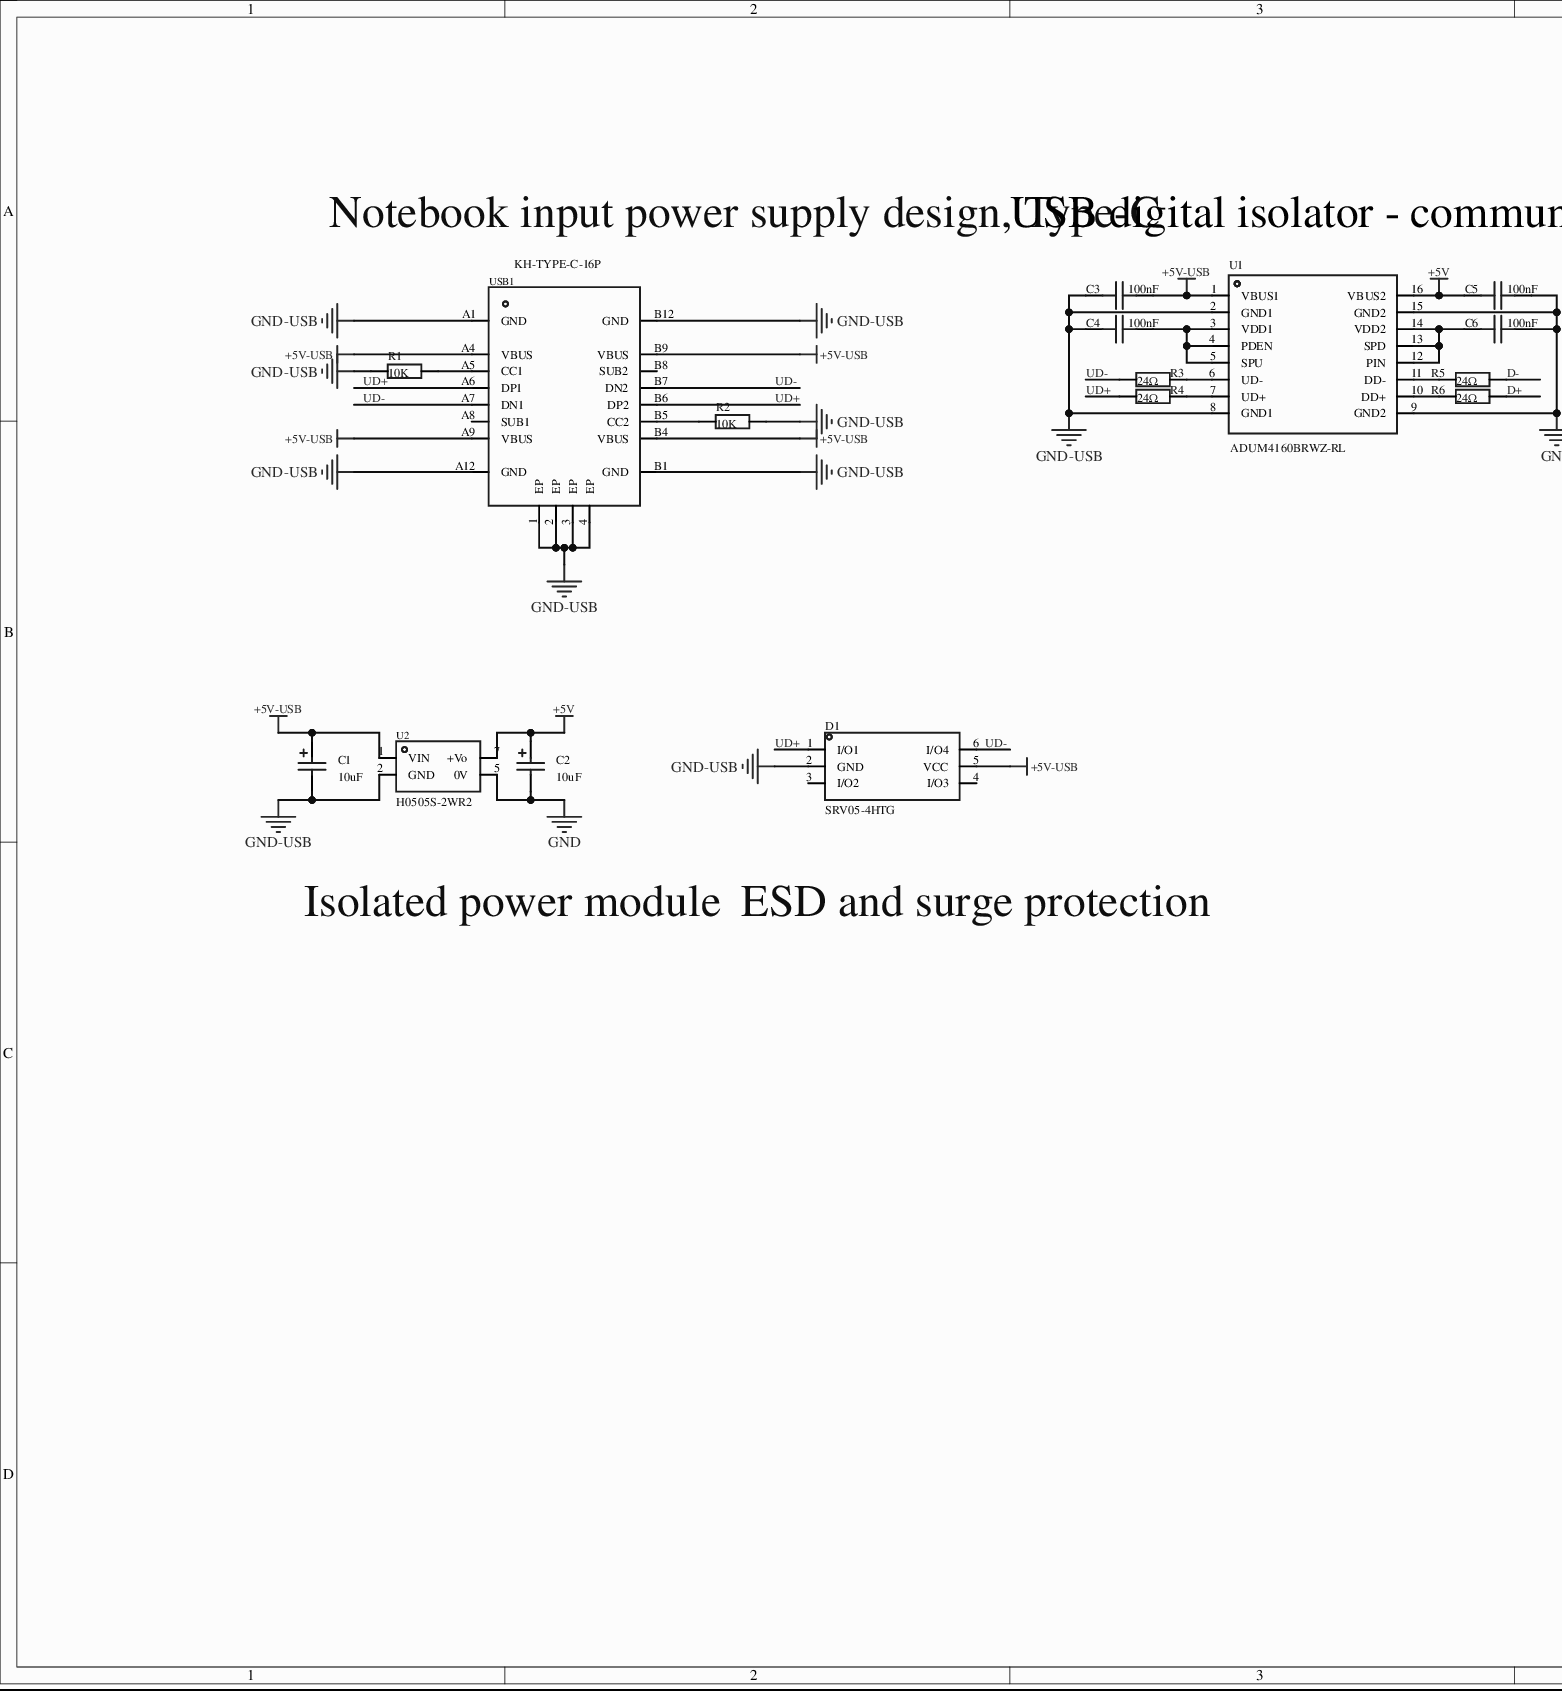
[diagram p0: MISC79005-3.schdoc, left]
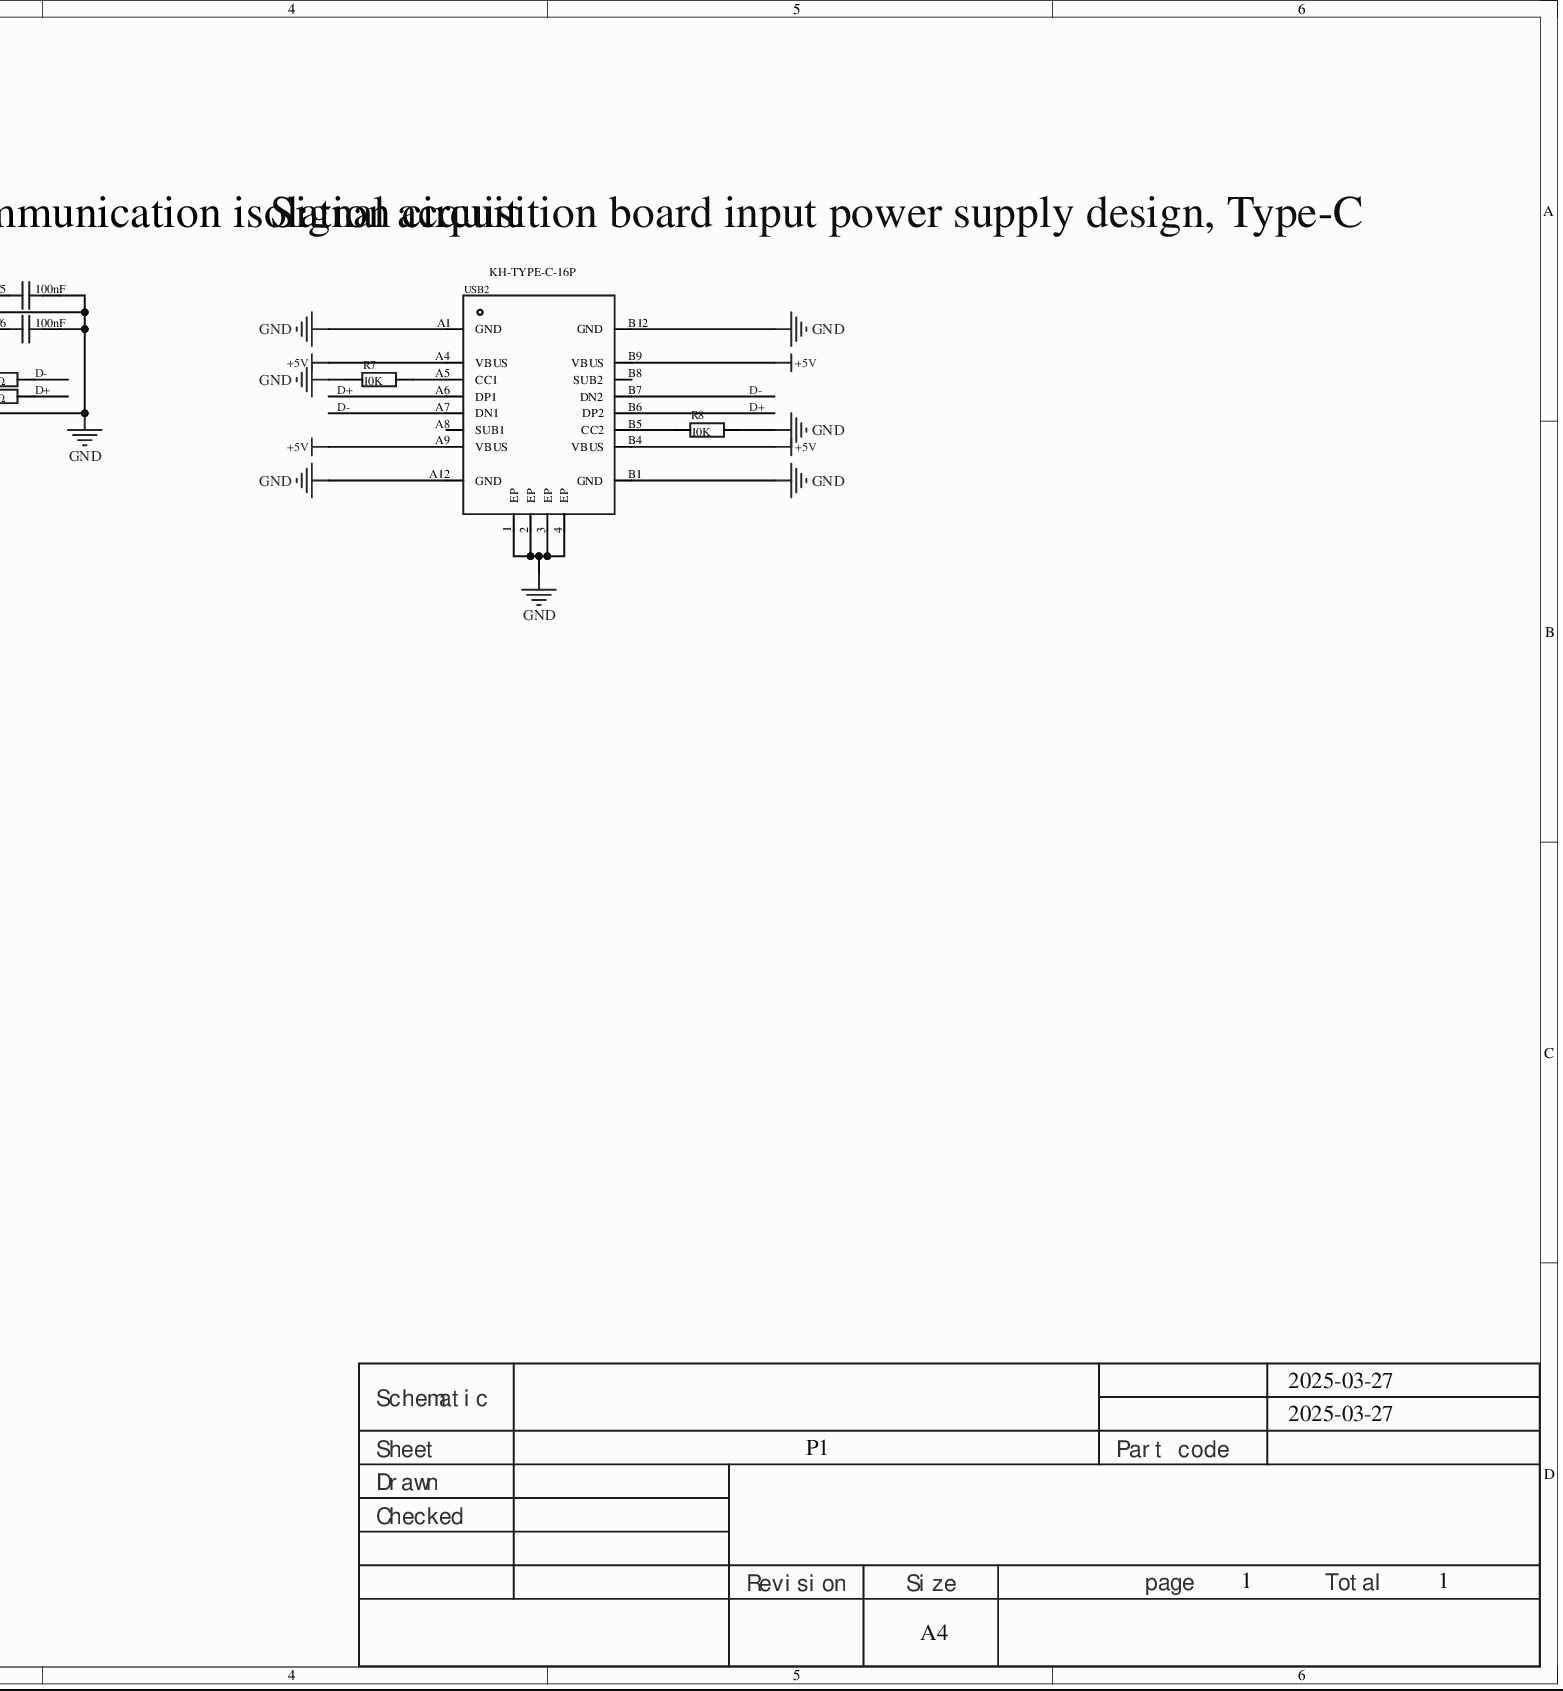
[diagram p1: MISC79005-3.schdoc, right]
# Altium project MISC79005-2.PrjPcb
1 sheet, 19 parts. Net scope: global (net labels, ports and power ports of the same name join across sheets).
Board file: MISC79005.pcbdoc

## Sheet MISC79005-3.schdoc
size 457 x 254 mm; Version: V1.0; @Project Name: MISC79005; @Page Count: 1; @Update Date: 2025-03-27; @Create Date: 2025-03-27; @Schematic Name: MISC79005; @Page No: 1; @Board Name: MISC79005; @Create Time: 09:58:40; @Update Time: 21:52:18

### Parts
C1  10uF  [CAP-SMD_L3.2-W1.6-RD-C7171]
C2  10uF  [CAP-SMD_L3.2-W1.6-RD-C7171]
C3  100nF  [C0603]
C4  100nF  [C0603]
C5  100nF  [C0603]
C6  100nF  [C0603]
D1  SRV05-4HTG  [SOT-23-6_L2.9-W1.6-P0.95-LS2.8-BL]
R1  10K  [R0603]
R2  10K  [R0603]
R3  24Ω  [R0603]
R4  24Ω  [R0603]
R5  24Ω  [R0603]
R6  24Ω  [R0603]
R7  10K  [R0603]
R8  10K  [R0603]
U1  ADUM4160BRWZ-RL  [SOIC-16_L10.3-W7.5-P1.27-LS10.3-BL]
U2  H0505S-2WR2  [PWRM-TH_EVISUN_HXXXXS-2WR2]
USB1  KH-TYPE-C-16P  [USB-C-SMD_KH-TYPE-C-16P]
USB2  KH-TYPE-C-16P  [USB-C-SMD_KH-TYPE-C-16P]

### Nets
+5V: C2.1 C5.1 U1.16(VBUS2) U2.7(+Vo) USB2.A4(VBUS) USB2.A9(VBUS) USB2.B4(VBUS) USB2.B9(VBUS)
+5V-USB: C1.1 C3.2 D1.5(VCC) U1.1(VBUS1) U2.1(VIN) USB1.A4(VBUS) USB1.A9(VBUS) USB1.B4(VBUS) USB1.B9(VBUS)
GND: C2.2 C5.2 C6.2 R7.2 R8.1 U1.9(GND2) U1.15(GND2) U2.5(0V) USB2.1(EP) USB2.2(EP) USB2.3(EP) USB2.4(EP) USB2.A1(GND) USB2.A12(GND) USB2.B1(GND) USB2.B12(GND)
GND-USB: C1.2 C3.1 C4.1 D1.2(GND) R1.2 R2.1 U1.2(GND1) U1.8(GND1) U2.2(GND) USB1.1(EP) USB1.2(EP) USB1.3(EP) USB1.4(EP) USB1.A1(GND) USB1.A12(GND) USB1.B1(GND) USB1.B12(GND)
D+: R6.2 USB2.A6(DP1) USB2.B6(DP2)
D-: R5.2 USB2.A7(DN1) USB2.B7(DN2)
UD+: D1.1(I/O1) R4.1 USB1.A6(DP1) USB1.B6(DP2)
UD-: D1.6(I/O4) R3.1 USB1.A7(DN1) USB1.B7(DN2)
NetC4_2: C4.2 U1.3(VDD1) U1.4(PDEN) U1.5(SPU)
NetC6_1: C6.1 U1.12(PIN) U1.13(SPD) U1.14(VDD2)
NetR1_1: R1.1 USB1.A5(CC1)
NetR2_2: R2.2 USB1.B5(CC2)
NetR3_2: R3.2 U1.6(UD-)
NetR4_2: R4.2 U1.7(UD+)
NetR5_1: R5.1 U1.11(DD-)
NetR6_1: R6.1 U1.10(DD+)
NetR7_1: R7.1 USB2.A5(CC1)
NetR8_2: R8.2 USB2.B5(CC2)

Not connected (* = marked no-connect by the designer): D1 3(I/O2)* 4(I/O3)*; USB1 A8(SUB1)* B8(SUB2)*; USB2 A8(SUB1)* B8(SUB2)*

### Notes on the sheet
- Notebook input power supply design, Type-C
- USB digital isolator - communication isolation circuit
- Signal acquisition board input power supply design, Type-C
- Isolated power module
- ESD and surge protection
- 2025-03-27
- Schematic
- Sheet
- P1
- Part code
- Checked
- Drawn
- Revision
- Size
- A4
- page
- 1
- Total

### Library data of the parts
C1 C2 = TAJA106K016RNJ: Capacitance: 10uF; Tolerance: ±10%; Rated voltage: 16V; ESR: 3Ω@100kHz;; Manufacturer: Kyocera AVX; AddInBom: yes; ModelId: d42b6f9952ad429a883ac5dd55ff7452; ModelName: CASE-A_L3.2-W1.6-H1.6; ModelTransform: 125.984,62.992,0,0,0,0,0,0,0; Device: TAJA106K016RNJ; Symbol: TAJA106K016RNJ; LCSC Part Name: 10uF ±10% 16V; SupplierPart: C7171; ManufacturerPart: TAJA106K016RNJ; Supplier Footprint: CASE-A-3216; Datasheet: https://example.com/upload/public/pdf/source/20160107/1457707748093.pdf; Supplier: LCSC; ConvertToPcb: yes; FootprintName: CAP-SMD_L3.2-W1.6-RD-C7171; Value: 10uF; Rated Voltage: 16V; Equivalent Series Resistance(ESR): 3Ω@100kHz; Operating Temperature: -55℃~+125℃
C3-C6 = CC0603KRX7R9BB104: Capacitance: 100nF; Tolerance: ±10%; Rated voltage: 50V; Dielectric (temperature coefficient): X7R;; Manufacturer: YAGEO(国巨); AddInBom: yes; ModelId: ac125912035d415993ca9572d50418b1; ModelName: C0603_L1.6-W0.8-H0.8; ModelTransform: 62.992,31.496,0,0,0,0,0,0,0; Value: 100nF; Device: CC0603KRX7R9BB104; Symbol: CC0603KRX7R9BB104; LCSC Part Name: 100nF±10%50V; SupplierPart: C14663; ManufacturerPart: CC0603KRX7R9BB104; Supplier Footprint: 0603; JLCPCB Part Class: Basic library; Datasheet: https://example.com/upload/public/pdf/source/20170116/1484561234239.pdf; Supplier: LCSC; ConvertToPcb: yes; FootprintName: C0603; Voltage Rated: 50V; Temperature Coefficient: X7R
D1 = SRV05-4HTG_C151305: Reverse stand-off voltage (Vrwm): 6V@Max; Breakdown voltage: -; Peak pulse current (Ipp)@10/1000μs: -; Max clamping voltage: 15V; Peak pulse power (Ppp)@10/1000μs: 150W;; Manufacturer: Littelfuse(美国力特); AddInBom: yes; ModelId: 18da8f6c14a34920b3e136b5c401a119; ModelName: SOT-23-6_L2.9-W1.6-H1.5-LS2.8-P0.95; ModelTransform: 110.236,113.364,0,90,0,0,0.0005,0.0005,0; Device: SRV05-4HTG_C151305; Symbol: SRV05-4HTG; LCSC Part Name: Vrwm:6V@Max 150W; SupplierPart: C151305; ManufacturerPart: SRV05-4HTG; Supplier Footprint: SOT-23-6; JLCPCB Part Class: Extended library; Datasheet: https://example.com/upload/public/pdf/source/20171201/C151305_15121210238401156993.pdf; Supplier: LCSC; ConvertToPcb: yes; FootprintName: SOT-23-6_L2.9-W1.6-P0.95-LS2.8-BL; Reverse Stand-Off Voltage (Vrwm): 6V@Max; Breakdown Voltage: -; Peak Pulse Current (Ipp)@10/1000μs: -; Maximum Clamping Voltage: 15V; Peak Pulse Power Dissipation (Ppp)@10/1000μs: 150W
R1 R2 R7 R8 = Res_0805: Symbol: Resistor; ConvertToPcb: yes; ModelId: 37a81e68749a4138bd2dfa6897b24b85; ModelName: R0805_L2.0-W1.3-H0.6; ModelTransform: 78.74,51.181,0,0,0,0,0,-0.0005,0; Device: Res_0805; AddInBom: yes; Supplier Footprint: 0805; Value: 10K; FootprintName: R0603
R3-R6 = RC0603FR-0724RL: Resistor type: thick-film resistor; Resistance: 24Ω; Tolerance: ±1%; Power: 100mW; Temperature coefficient: ±100ppm/℃; Max working voltage: 75V; Operating temperature range: -55℃~+155℃;; Manufacturer: YAGEO(国巨); AddInBom: yes; ModelId: 3281a289d46d4bb1877be1eabd090e13; ModelName: R0603_L1.6-W0.8-H0.8; ModelTransform: 62.992,31.496,0,0,0,0,0,0,0; Device: RC0603FR-0724RL; Symbol: RC0603FR-0724RL; LCSC Part Name: 24Ω±1%100mW; SupplierPart: C137758; ManufacturerPart: RC0603FR-0724RL; Supplier Footprint: 0603; JLCPCB Part Class: Extended library; Datasheet: https://example.com/upload/public/pdf/source/20171106/C137758_15099606446381093894.pdf; Supplier: LCSC; ConvertToPcb: yes; FootprintName: R0603; Type: Thick-film resistor; Value: 24Ω; Power(Watts): 100mW; Temperature Coefficient: ±100ppm/℃; Overload Voltage (Max): 75V; Operating Temperature Range: -55℃~+155℃
U1 = ADUM4160BRWZ-RL_C57791: Isolator technology: Magnetic Coupling; Type: USB; Channels: 1; Channel type: Bidirectional; Isolation voltage: 5000Vrms; Data rate: 12Mbps;; Manufacturer: ADI(亚德诺)/LINEAR(凌特); AddInBom: yes; ModelId: 2da8125c657e49328ba6fa7b098653dd; ModelName: SOIC-16_L10.3-W7.5-H2.7-LS10.3-P1.27; ModelTransform: 405.511,409.68154,0,0,0,0,-0.0005,0,0; Isolated Power: No; Number of Channels: 1; Inputs - Side 1/Side 2: 2/2; Voltage - Supply: 3.1V~5.5V; Device: ADUM4160BRWZ-RL_C57791; Symbol: ADUM4160BRWZ; LCSC Part Name: ADUM4160BRWZ-RL; SupplierPart: C57791; ManufacturerPart: ADUM4160BRWZ-RL; Supplier Footprint: SOIC-16_300mil; JLCPCB Part Class: Extended library; Datasheet: https://example.com/upload/public/pdf/source/20180327/C57791_1A1DC0BD2A9501538E79ECF10A1F69DF.pdf; Supplier: LCSC; ConvertToPcb: yes; FootprintName: SOIC-16_L10.3-W7.5-P1.27-LS10.3-BL; Technology: MagneticCoupling; Channel Type: Bidirectional; Voltage - Isolation: 5000Vrms; Data Rate: 12Mbps
U2 = H0505S-2WR2: Converter type: DC-DC; Input voltage (DC): 4.5V~5.5V; Output voltage: 5V; Output current (max): 400mA; Output power: 2W; Efficiency: 88%;; Manufacturer: EVISUN(易成); AddInBom: yes; ModelId: 15c6874ec71d411289e402ccc028a224; ModelTransform: 767.715,386.22,0,0,0,0,0,-82.677,-157.48; Symbol: H0505S-2WR2; Device: H0505S-2WR2; Supplier: LCSC; Supplier Part: C7598646; Manufacturer Part: H0505S-2WR2; LCSC Part Name: DC/DC直流转直流隔离6000Vdc电源模块5V转5V400mA; Supplier Footprint: SIP-4; Datasheet: https://example.com/upload/public/pdf/source/20230906/8FA7DC7AB23272A2B5783D76087F325F.pdf; ConvertToPcb: yes; FootprintName: PWRM-TH_EVISUN_HXXXXS-2WR2; ModelName: PWRM-TH_EVISUN_HXXXXS-2WR2; Conversion Type: DC-DC; Input Voltage(DC): 4.5V~5.5V; Output Voltage: 5V; Output Current (Max): 400mA; Output Power: 2W; Conversion Efficiency: 88%
USB1 USB2 = KH-TYPE-C-16P: Type-C receptacle 16PIN, vertical, four-corner SMT, no hold-down tabs; Manufacturer: kinghelm(金航标); AddInBom: yes; ModelId: f2c381012fbf47e0b76dea5162270f01; ModelTransform: 351.9678,307.48,0,0,0,0,0,-45.275,-43.307; Symbol: KH-TYPE-C-16P; Device: KH-TYPE-C-16P; Supplier: LCSC; Supplier Part: C709357; Manufacturer Part: KH-TYPE-C-16P; JLCPCB Part Class: Extended library; LCSC Part Name: Type-C母座; Supplier Footprint: -; ConvertToPcb: yes; FootprintName: USB-C-SMD_KH-TYPE-C-16P; ModelName: USB-C-SMD_KH-TYPE-C-16P